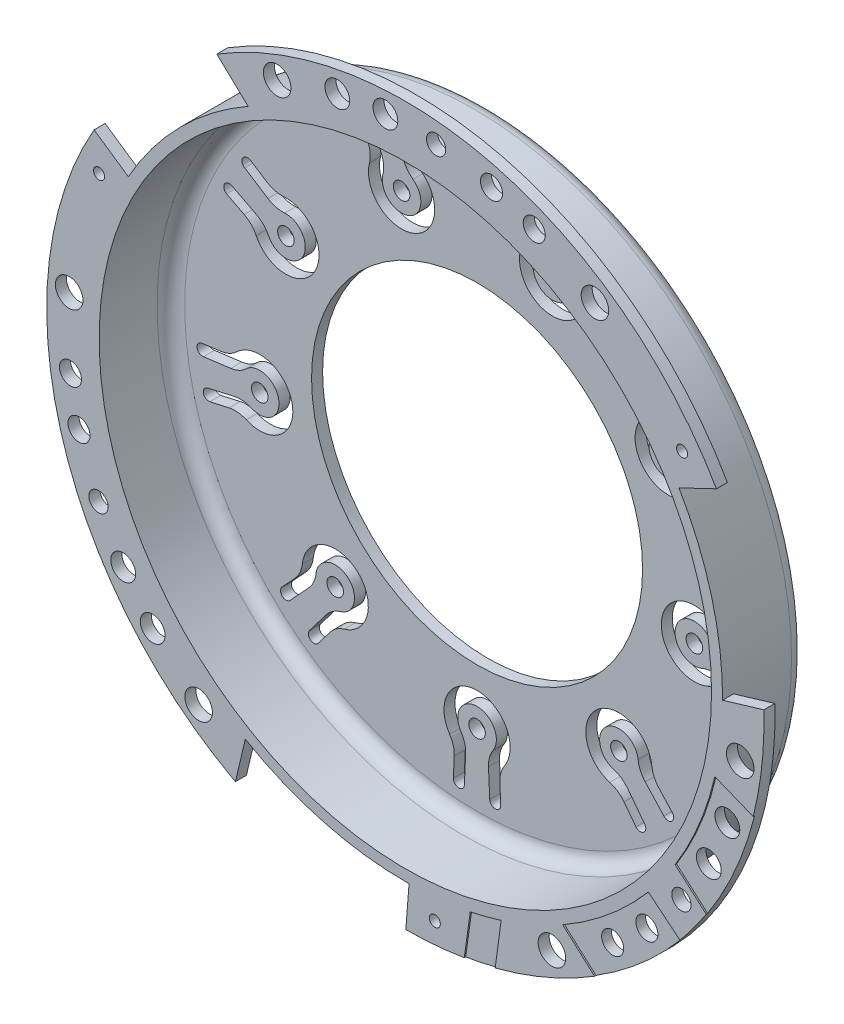
SolidWorks part; units mm, degrees
ref_plane "Front Plane" through (0, 0, 0) normal (0, 0, 1) x (1, 0, 0)
ref_plane "Top Plane" through (0, 0, 0) normal (0, 1, 0) x (1, 0, 0)
ref_plane "Right Plane" through (0, 0, 0) normal (1, 0, 0) x (0, 0, -1)
other "Configuration Table"
sketch "Sketch1" plane through (0, 0, 0) normal (0, 0, 1) x (1, 0, 0)
  circle A0 centre (0, 0) radius 115
extrude "Boss-Extrude1" add sketch "Sketch1" along normal blind 30
shell "Shell1" thickness 4
fillet "Fillet1" radius 5 1 edges at (115, 0, 0)
fillet "Fillet2" radius 5 1 edges at (111, 0, 4)
sketch "Sketch2" plane through (0, 0, 30) normal (0, 0, 1) x (1, 0, 0)
  circle A0 centre (0, 0) radius 130
  circle A1 centre (0, 0) radius 115 construction
  circle A2 centre (0, 0) radius 115
extrude "Boss-Extrude2" add sketch "Sketch2" against normal blind 4
sketch "Sketch3" plane through (0, 0, 4) normal (0, 0, 1) x (1, 0, 0)
  circle A0 centre (0, 0) radius 60
extrude "Cut-Extrude1" cut sketch "Sketch3" against normal through all
sketch "Sketch4" plane through (0, 0, 4) normal (0, 0, 1) x (1, 0, 0)
  line L0 (4.5928, -99.8945) -> (4.1343, -89.9208)
  line L1 (-4.5928, -99.8945) -> (-4.1343, -89.9208)
  line L2 (8.5928, -99.8945) -> (8.2673, -92.7349)
  line L3 (-8.5928, -99.8945) -> (-8.2673, -92.7349)
  line L4 (0, 0) -> (0, -92.6549) construction
  line L5 (-60.6926, -79.4758) -> (-54.6329, -71.5408)
  line L6 (-67.7293, -73.5714) -> (-60.967, -66.2259)
  line L7 (-57.6284, -82.047) -> (-53.2757, -76.3532)
  line L8 (-70.7934, -71.0002) -> (-65.942, -65.7249)
  line L9 (-97.5793, -21.8696) -> (-87.8368, -19.6861)
  line L10 (-99.1744, -12.8234) -> (-89.2726, -11.5431)
  line L11 (-96.8847, -25.8088) -> (-89.8904, -24.245)
  line L12 (-99.869, -8.8842) -> (-92.7616, -7.9615)
  line L13 (-88.8076, 45.9697) -> (-79.9408, 41.38)
  line L14 (-84.2147, 53.9248) -> (-75.8065, 48.5408)
  line L15 (-90.8076, 42.5056) -> (-84.4444, 39.2077)
  line L16 (-82.2147, 57.3889) -> (-76.1771, 53.5272)
  line L17 (-38.4818, 92.2993) -> (-34.6397, 83.0839)
  line L18 (-29.8501, 95.4409) -> (-26.8698, 85.9119)
  line L19 (-42.2406, 90.9312) -> (-39.4859, 84.3147)
  line L20 (-26.0913, 96.809) -> (-23.9485, 89.9699)
  line L21 (29.8501, 95.4409) -> (26.8698, 85.9119)
  line L22 (38.4818, 92.2993) -> (34.6397, 83.0839)
  line L23 (26.0913, 96.809) -> (23.9485, 89.9699)
  line L24 (42.2406, 90.9312) -> (39.4859, 84.3147)
  line L25 (84.2147, 53.9248) -> (75.8065, 48.5408)
  line L26 (88.8076, 45.9697) -> (79.9408, 41.38)
  line L27 (82.2147, 57.3889) -> (76.1771, 53.5272)
  line L28 (90.8076, 42.5056) -> (84.4444, 39.2077)
  line L29 (99.1744, -12.8234) -> (89.2726, -11.5431)
  line L30 (97.5793, -21.8696) -> (87.8368, -19.6861)
  line L31 (99.869, -8.8842) -> (92.7616, -7.9615)
  line L32 (96.8847, -25.8088) -> (89.8904, -24.245)
  line L33 (67.7293, -73.5714) -> (60.967, -66.2259)
  line L34 (60.6926, -79.4758) -> (54.6329, -71.5408)
  line L35 (70.7934, -71.0002) -> (65.942, -65.7249)
  line L36 (57.6284, -82.047) -> (53.2757, -76.3532)
  circle A0 centre (0, 0) radius 80 construction
  arc A1 (5.8157, -83.8959) -> (-5.8157, -83.8959) centre (0, -80) ccw
  arc A2 (5.8157, -83.8959) -> (4.1343, -89.9208) centre (14.1237, -89.4615) ccw
  arc A3 (-4.1343, -89.9208) -> (-5.8157, -83.8959) centre (-14.1237, -89.4615) ccw
  arc A4 (9.9582, -86.6958) -> (-9.9582, -86.6958) centre (0, -80) ccw
  arc A5 (9.9582, -86.6958) -> (8.2673, -92.7349) centre (18.2568, -92.2756) ccw
  arc A6 (-8.2673, -92.7349) -> (-9.9582, -86.6958) centre (-18.2568, -92.2756) ccw
  arc A7 (4.5928, -99.8945) -> (8.5928, -99.8945) centre (6.5928, -99.8945) ccw
  arc A8 (-8.5928, -99.8945) -> (-4.5928, -99.8945) centre (-6.5928, -99.8945) ccw
  circle A9 centre (0, -80) radius 3
  arc A10 (-49.4722, -68.0062) -> (-58.3823, -60.5298) centre (-51.423, -61.2836) ccw
  arc A11 (-49.4722, -68.0062) -> (-54.6329, -71.5408) centre (-46.6853, -77.6101) ccw
  arc A12 (-60.967, -66.2259) -> (-58.3823, -60.5298) centre (-68.3242, -59.4529) ccw
  arc A13 (-48.0985, -72.8139) -> (-63.3554, -60.0118) centre (-51.423, -61.2836) ccw
  arc A14 (-48.0985, -72.8139) -> (-53.2757, -76.3532) centre (-45.3281, -82.4224) ccw
  arc A15 (-65.942, -65.7249) -> (-63.3554, -60.0118) centre (-73.2991, -58.952) ccw
  arc A16 (-60.6926, -79.4758) -> (-57.6284, -82.047) centre (-59.1605, -80.7614) ccw
  arc A17 (-70.7934, -71.0002) -> (-67.7293, -73.5714) centre (-69.2613, -72.2858) ccw
  circle A18 centre (-51.423, -61.2836) radius 3
  arc A19 (-81.6115, -20.2957) -> (-83.6312, -8.8411) centre (-78.7846, -13.8919) ccw
  arc A20 (-81.6115, -20.2957) -> (-87.8368, -19.6861) centre (-85.6498, -29.444) ccw
  arc A21 (-89.2726, -11.5431) -> (-83.6312, -8.8411) centre (-90.5549, -1.6257) ccw
  arc A22 (-83.6494, -24.8615) -> (-87.1079, -5.2476) centre (-78.7846, -13.8919) ccw
  arc A23 (-83.6494, -24.8615) -> (-89.8904, -24.245) centre (-87.7035, -34.0029) ccw
  arc A24 (-92.7616, -7.9615) -> (-87.1079, -5.2476) centre (-94.044, 1.9559) ccw
  arc A25 (-97.5793, -21.8696) -> (-96.8847, -25.8088) centre (-97.232, -23.8392) ccw
  arc A26 (-99.869, -8.8842) -> (-99.1744, -12.8234) centre (-99.5217, -10.8538) ccw
  circle A27 centre (-78.7846, -13.8919) radius 3
  arc A28 (-75.5638, 36.9115) -> (-69.7482, 46.9845) centre (-69.282, 40) ccw
  arc A29 (-75.5638, 36.9115) -> (-79.9408, 41.38) centre (-84.5378, 32.4992) ccw
  arc A30 (-75.8065, 48.5408) -> (-69.7482, 46.9845) centre (-70.4141, 56.9623) ccw
  arc A31 (-80.0599, 34.7238) -> (-70.1016, 51.972) centre (-69.282, 40) ccw
  arc A32 (-80.0599, 34.7238) -> (-84.4444, 39.2077) centre (-89.0414, 30.327) ccw
  arc A33 (-76.1771, 53.5272) -> (-70.1016, 51.972) centre (-70.7846, 61.9486) ccw
  arc A34 (-88.8076, 45.9697) -> (-90.8076, 42.5056) centre (-89.8076, 44.2377) ccw
  arc A35 (-82.2147, 57.3889) -> (-84.2147, 53.9248) centre (-83.2147, 55.6568) ccw
  circle A36 centre (-69.282, 40) radius 3
  arc A37 (-34.159, 76.8473) -> (-23.2292, 80.8254) centre (-27.3616, 75.1754) ccw
  arc A38 (-34.159, 76.8473) -> (-34.6397, 83.0839) centre (-43.8696, 79.2357) ccw
  arc A39 (-26.8698, 85.9119) -> (-23.2292, 80.8254) centre (-17.3257, 88.8969) ccw
  arc A40 (-39.0094, 78.0615) -> (-20.294, 84.8733) centre (-27.3616, 75.1754) ccw
  arc A41 (-39.0094, 78.0615) -> (-39.4859, 84.3147) centre (-48.7159, 80.4665) ccw
  arc A42 (-23.9485, 89.9699) -> (-20.294, 84.8733) centre (-14.4044, 92.9549) ccw
  arc A43 (-38.4818, 92.2993) -> (-42.2406, 90.9312) centre (-40.3612, 91.6152) ccw
  arc A44 (-26.0913, 96.809) -> (-29.8501, 95.4409) centre (-27.9707, 96.125) ccw
  circle A45 centre (-27.3616, 75.1754) radius 3
  arc A46 (23.2292, 80.8254) -> (34.159, 76.8473) centre (27.3616, 75.1754) ccw
  arc A47 (23.2292, 80.8254) -> (26.8698, 85.9119) centre (17.3257, 88.8969) ccw
  arc A48 (34.6397, 83.0839) -> (34.159, 76.8473) centre (43.8696, 79.2357) ccw
  arc A49 (20.294, 84.8733) -> (39.0094, 78.0615) centre (27.3616, 75.1754) ccw
  arc A50 (20.294, 84.8733) -> (23.9485, 89.9699) centre (14.4044, 92.9549) ccw
  arc A51 (39.4859, 84.3147) -> (39.0094, 78.0615) centre (48.7159, 80.4665) ccw
  arc A52 (29.8501, 95.4409) -> (26.0913, 96.809) centre (27.9707, 96.125) ccw
  arc A53 (42.2406, 90.9312) -> (38.4818, 92.2993) centre (40.3612, 91.6152) ccw
  circle A54 centre (27.3616, 75.1754) radius 3
  arc A55 (69.7482, 46.9845) -> (75.5638, 36.9115) centre (69.282, 40) ccw
  arc A56 (69.7482, 46.9845) -> (75.8065, 48.5408) centre (70.4141, 56.9623) ccw
  arc A57 (79.9408, 41.38) -> (75.5638, 36.9115) centre (84.5378, 32.4992) ccw
  arc A58 (70.1016, 51.972) -> (80.0599, 34.7238) centre (69.282, 40) ccw
  arc A59 (70.1016, 51.972) -> (76.1771, 53.5272) centre (70.7846, 61.9486) ccw
  arc A60 (84.4444, 39.2077) -> (80.0599, 34.7238) centre (89.0414, 30.327) ccw
  arc A61 (84.2147, 53.9248) -> (82.2147, 57.3889) centre (83.2147, 55.6568) ccw
  arc A62 (90.8076, 42.5056) -> (88.8076, 45.9697) centre (89.8076, 44.2377) ccw
  circle A63 centre (69.282, 40) radius 3
  arc A64 (83.6312, -8.8411) -> (81.6115, -20.2957) centre (78.7846, -13.8919) ccw
  arc A65 (83.6312, -8.8411) -> (89.2726, -11.5431) centre (90.5549, -1.6257) ccw
  arc A66 (87.8368, -19.6861) -> (81.6115, -20.2957) centre (85.6498, -29.444) ccw
  arc A67 (87.1079, -5.2476) -> (83.6494, -24.8615) centre (78.7846, -13.8919) ccw
  arc A68 (87.1079, -5.2476) -> (92.7616, -7.9615) centre (94.044, 1.9559) ccw
  arc A69 (89.8904, -24.245) -> (83.6494, -24.8615) centre (87.7035, -34.0029) ccw
  arc A70 (99.1744, -12.8234) -> (99.869, -8.8842) centre (99.5217, -10.8538) ccw
  arc A71 (96.8847, -25.8088) -> (97.5793, -21.8696) centre (97.232, -23.8392) ccw
  circle A72 centre (78.7846, -13.8919) radius 3
  arc A73 (58.3823, -60.5298) -> (49.4722, -68.0062) centre (51.423, -61.2836) ccw
  arc A74 (58.3823, -60.5298) -> (60.967, -66.2259) centre (68.3242, -59.4529) ccw
  arc A75 (54.6329, -71.5408) -> (49.4722, -68.0062) centre (46.6853, -77.6101) ccw
  arc A76 (63.3554, -60.0118) -> (48.0985, -72.8139) centre (51.423, -61.2836) ccw
  arc A77 (63.3554, -60.0118) -> (65.942, -65.7249) centre (73.2991, -58.952) ccw
  arc A78 (53.2757, -76.3532) -> (48.0985, -72.8139) centre (45.3281, -82.4224) ccw
  arc A79 (67.7293, -73.5714) -> (70.7934, -71.0002) centre (69.2613, -72.2858) ccw
  arc A80 (57.6284, -82.047) -> (60.6926, -79.4758) centre (59.1605, -80.7614) ccw
  circle A81 centre (51.423, -61.2836) radius 3
  point P187 (0, 0)
  dimension "D1" = 9
extrude "Cut-Extrude2" cut sketch "Sketch4" against normal through all
sketch "Sketch5" plane through (0, 0, 30) normal (0, 0, 1) x (1, 0, 0)
  circle A0 centre (0, 0) radius 115
  circle A1 centre (0, 0) radius 147.9633
extrude "Cut-Extrude3" cut sketch "Sketch5" against normal through all
sketch "Sketch6" plane through (0, 0, 30) normal (0, 0, 1) x (1, 0, 0)
  line L0 (1.3424, -114.9787) -> (0.1768, -129.9999)
  line L1 (114.9985, -0.5832) -> (129.942, 3.884)
  arc A0 (0.1768, -129.9999) -> (129.942, 3.884) centre (0, 0) ccw
  circle A1 centre (10.6951, -122.0204) radius 2
  circle A2 centre (0, 0) radius 122.5 construction
  circle A3 centre (109.5202, -54.8779) radius 4.5
  circle A4 centre (87.0598, -86.33) radius 4
  circle A5 centre (53.126, -110.0492) radius 5
  circle A6 centre (74.6554, -97.0627) radius 4
  circle A7 centre (100.0704, -70.6552) radius 3.5
  circle A8 centre (121.3927, -16.4339) radius 5
  circle A9 centre (116.2447, -38.6448) radius 4.5
  arc A10 (1.3413, -114.9922) -> (114.9985, -0.5832) centre (0, 0) ccw
  circle M2 centre (0, 0) radius 115
extrude "Boss-Extrude3" add sketch "Sketch6" against normal blind 4 contours L0 A0 L1 A9 A8 A7 A6 A5 A4 A3 A1 M2
sketch "Sketch8" plane through (0, 0, 30) normal (0, 0, 1) x (1, 0, 0)
  line L0 (23.5372, -112.7391) -> (21.3565, -128.2338)
  line L1 (34.7265, -109.8097) -> (32.5676, -125.8545)
  line L2 (57.0314, -100.0576) -> (68.6049, -110.4236)
  line L3 (97.818, -60.7926) -> (109.0771, -70.7262)
  line L4 (88.0704, -74.214) -> (99.5388, -83.6183)
  line L5 (112.2061, -25.9595) -> (126.1117, -31.5568)
  arc A0 (22.4556, -120.4242) -> (33.6532, -117.7867) centre (0, 0) ccw construction
  arc A1 (23.5372, -112.7391) -> (34.7265, -109.8097) centre (0, 0) ccw
  arc A2 (21.3565, -128.2338) -> (32.5676, -125.8545) centre (0, 0) ccw
  arc A3 (57.0314, -100.0576) -> (88.0704, -74.214) centre (0, 0) ccw
  arc A4 (62.769, -105.1965) -> (93.7389, -78.8623) centre (0, 0) ccw construction
  arc A5 (68.6049, -110.4236) -> (99.5388, -83.6183) centre (0, 0) ccw
  arc A6 (97.818, -60.7926) -> (112.2061, -25.9595) centre (0, 0) ccw
  arc A7 (103.3873, -65.7063) -> (119.0838, -28.7279) centre (0, 0) ccw construction
  arc A8 (109.0771, -70.7262) -> (126.1117, -31.5568) centre (0, 0) ccw
extrude "Cut-Extrude4" cut sketch "Sketch8" against normal blind 0.5
sketch "Sketch9" plane through (0, 0, 30) normal (0, 0, 1) x (1, 0, 0)
  line L0 (-58.0043, -99.3) -> (-61.6074, -114.475)
  line L1 (-100.4061, 56.068) -> (-112.8235, 64.5822)
  line L2 (99.196, 58.1821) -> (112.7703, 64.675)
  line L3 (-56.9942, 99.8833) -> (-68.3346, 110.5911)
  arc A0 (-112.8235, 64.5822) -> (-61.6074, -114.475) centre (0, 0) ccw
  circle A1 centre (0, 0) radius 122.5 construction
  circle A2 centre (-111.2244, -51.3359) radius 3.5
  circle A3 centre (-74.9285, -96.9122) radius 5
  circle A4 centre (-102.2857, -67.4083) radius 4.5
  circle A5 centre (-91.5897, -81.3485) radius 4.5
  circle A6 centre (-121.3864, -16.1221) radius 4
  circle A7 centre (-118.2938, -32.231) radius 4
  circle A8 centre (-121.8684, 9.0161) radius 5
  arc A9 (112.7703, 64.675) -> (-68.3346, 110.5911) centre (0, 0) ccw
  circle A10 centre (-111.0203, 51.748) radius 2
  circle A11 centre (100.3252, 70.2724) radius 2
  circle A12 centre (46.7311, 113.1848) radius 4
  circle A13 centre (-46.4642, 113.3461) radius 5
  circle A14 centre (-7.2344, 122.2862) radius 4.5
  circle A15 centre (-24.655, 119.9933) radius 4.5
  circle A16 centre (11.154, 121.9911) radius 3.5
  circle A17 centre (31.2341, 118.561) radius 4
  circle A18 centre (68.7424, 101.0331) radius 5
  arc A19 (114.9985, -0.5832) -> (1.3413, -114.9922) centre (0, 0) ccw construction
  arc A20 (99.196, 58.1821) -> (-56.9942, 99.8833) centre (0, 0) ccw
  arc A21 (-100.4061, 56.068) -> (-58.0043, -99.3) centre (0, 0) ccw
extrude "Boss-Extrude4" add sketch "Sketch9" against normal blind 4
